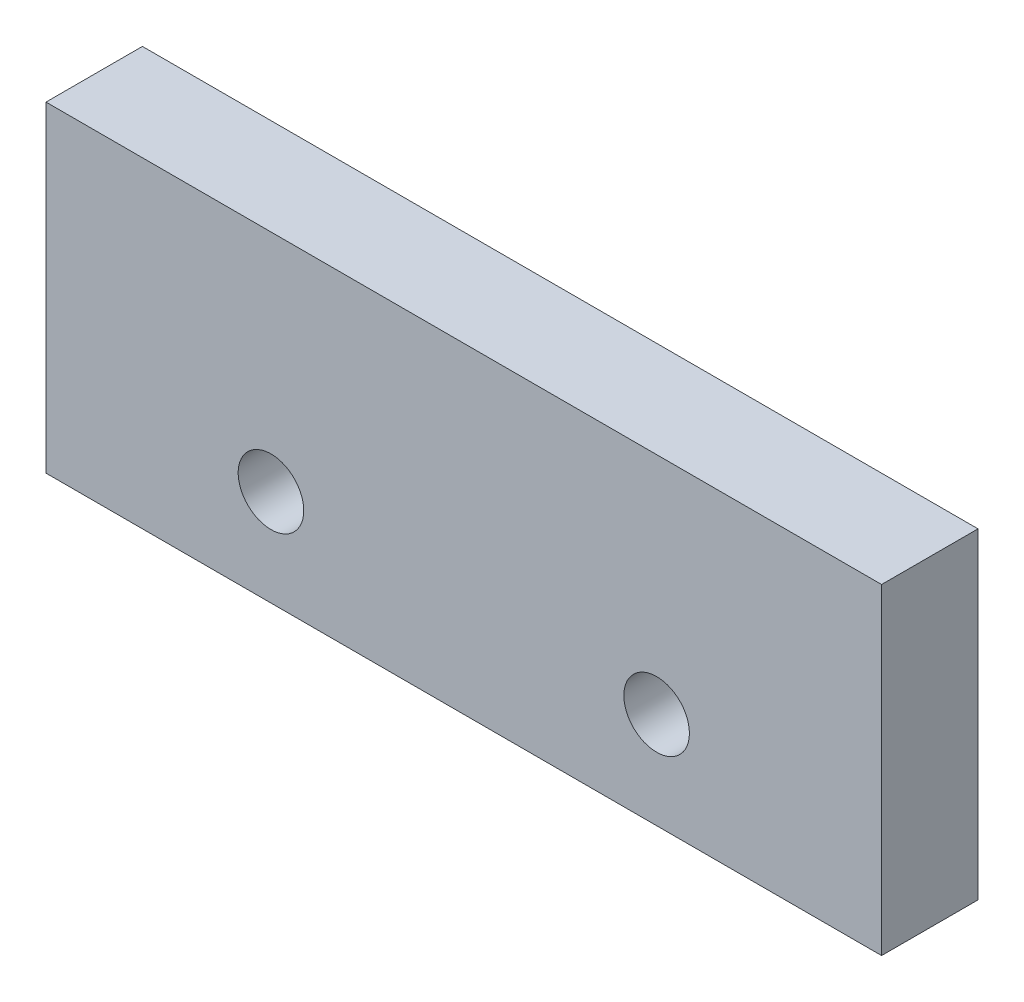
from build123d import *

# Parameters (mm, degrees)
SKETCH1_W              = 130
SKETCH1_H              = 50
BOSS_EXTRUDE1_DEPTH    = 15
M12_TAPPED_HOLE1_D     = 10.2
M12_TAPPED_HOLE1_DEPTH = 29.25
M12_TAPPED_HOLE1_TIP   = 3.064389157


with BuildPart() as part:
    # Sketch1 → Boss-Extrude1 (new body)
    with BuildSketch(Plane.XY):
        Rectangle(SKETCH1_W, SKETCH1_H)
    extrude(amount=BOSS_EXTRUDE1_DEPTH)

    # M12 Tapped Hole1
    with Locations(Plane.XY.offset(15)):
        with Locations((-30, -10), (30, -10)):
            Hole(M12_TAPPED_HOLE1_D / 2, depth=M12_TAPPED_HOLE1_DEPTH)
            with Locations((0, 0, -(M12_TAPPED_HOLE1_DEPTH + M12_TAPPED_HOLE1_TIP / 2))):  # 118° drill point
                Cone(0, M12_TAPPED_HOLE1_D / 2, M12_TAPPED_HOLE1_TIP, mode=Mode.SUBTRACT)


solid = part.part
